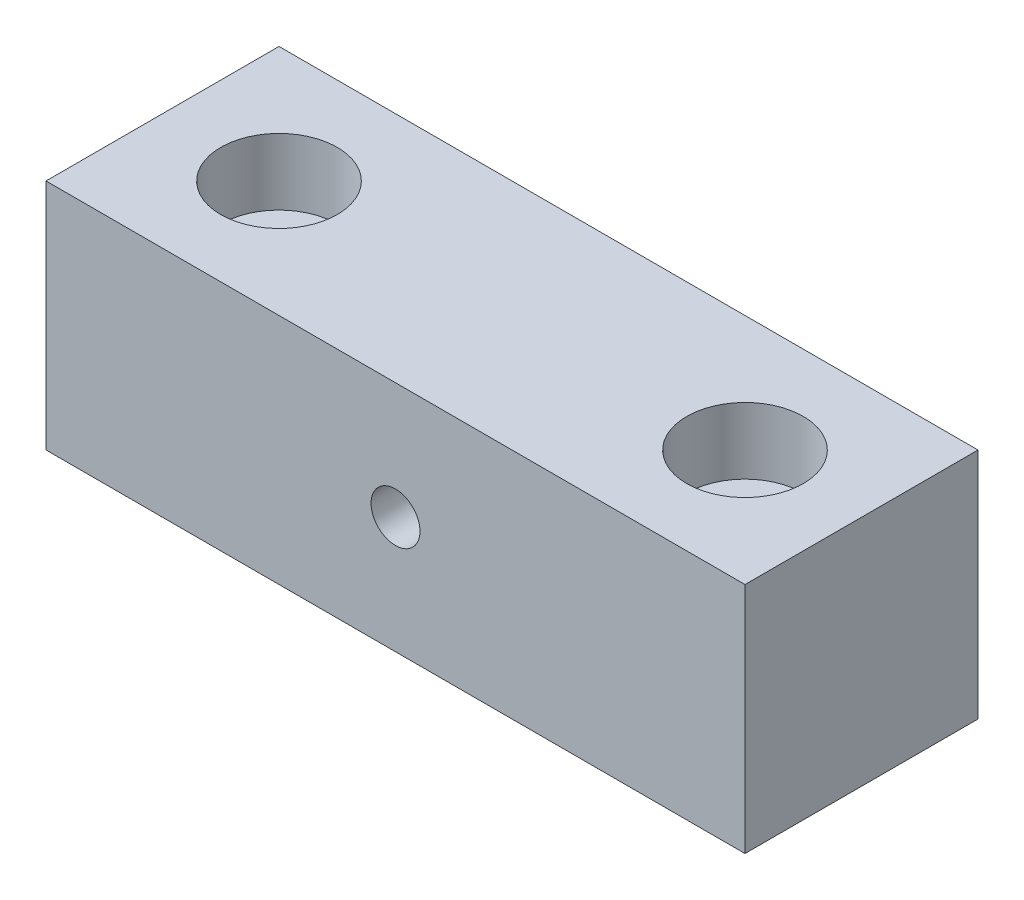
SolidWorks part; units mm, degrees
material "6061"
ref_plane "前视基准面" through (0, 0, 0) normal (0, 0, 1) x (1, 0, 0)
ref_plane "上视基准面" through (0, 0, 0) normal (0, 1, 0) x (1, 0, 0)
ref_plane "右视基准面" through (0, 0, 0) normal (1, 0, 0) x (0, 0, -1)
sketch "草图1" plane through (0, 0, 0) normal (0, 1, 0) x (1, 0, 0)
  line L1 (-30, -10) -> (30, -10)
  line L2 (-30, -10) -> (-30, 10)
  line L3 (-30, 10) -> (30, 10)
  line L4 (30, -10) -> (30, 10)
  line L5 (-30, -10) -> (30, 10) construction
  line L6 (-30, 10) -> (30, -10) construction
  point P0 (0, 0)
  dimension "D1" = 20
  dimension "D2" = 60
extrude "凸台-拉伸1" add sketch "草图1" along normal mid plane 20
hole_wizard "打孔尺寸(%根据)内六角圆柱头螺钉的类型1" positions "草图2" profile "草图3" counterbore size "M5" standard "GB" end condition through all
sketch "草图2" plane through (0, 10, 0) normal (0, 1, 0) x (1, 0, 0)
  line L0 (30, 0) -> (-30, 0) construction
  line L1 (30, -10) -> (30, 10) construction
  line L2 (-30, 10) -> (-30, -10) construction
  line L4 (0, 10) -> (0, -10) construction
  line L5 (30, 10) -> (-30, 10) construction
  line L6 (-30, -10) -> (30, -10) construction
  point P0 (20, 0)
  point P2 (-20, 0)
  dimension "D1" = 40
sketch "草图3" plane through (20, 10, 0) normal (1, 0, 0) x (0, 0, 1)
  line L0 (0, 0) -> (0, 20)
  line L1 (0, 20) -> (2.75, 20)
  line L3 (2.75, 20) -> (2.75, 5.7)
  line L4 (2.75, 5.7) -> (5, 5.7)
  line L5 (5, 5.7) -> (5, 0)
  line L7 (5, 0) -> (0, 0)
  line L11 (0, -6.35) -> (0, 107.95) construction
  dimension "通孔孔直径" = 5.5
  dimension "通孔孔深度" = 20
  dimension "柱形沉头孔直径" = 10
  dimension "柱形沉头孔深度" = 5.7
hole_wizard "M5 螺纹孔1" positions "草图4" profile "草图5" tap size "M5" standard "GB" end condition through all
sketch "草图4" plane through (0, 0, 10) normal (0, 0, 1) x (1, 0, 0)
  line L0 (30, 0) -> (-30, 0) construction
  line L1 (30, 10) -> (30, -10) construction
  line L2 (-30, 10) -> (-30, -10) construction
  line L4 (0, 10) -> (0, -10) construction
  line L5 (-30, 10) -> (30, 10) construction
  line L6 (-30, -10) -> (30, -10) construction
  point P0 (0, 0)
sketch "草图5" plane through (0, 0, 10) normal (1, 0, 0) x (0, -1, 0)
  line L0 (0, 0) -> (0, 20)
  line L1 (0, 20) -> (2.1, 20)
  line L2 (2.1, 20) -> (2.1, 0)
  line L5 (2.1, 0) -> (0, 0)
  line L11 (0, -6.35) -> (0, 107.95) construction
  dimension "通孔螺纹孔钻头直径" = 4.2
  dimension "通孔螺纹孔钻头深度" = 20
cosmetic thread "孔螺蚊线1"
